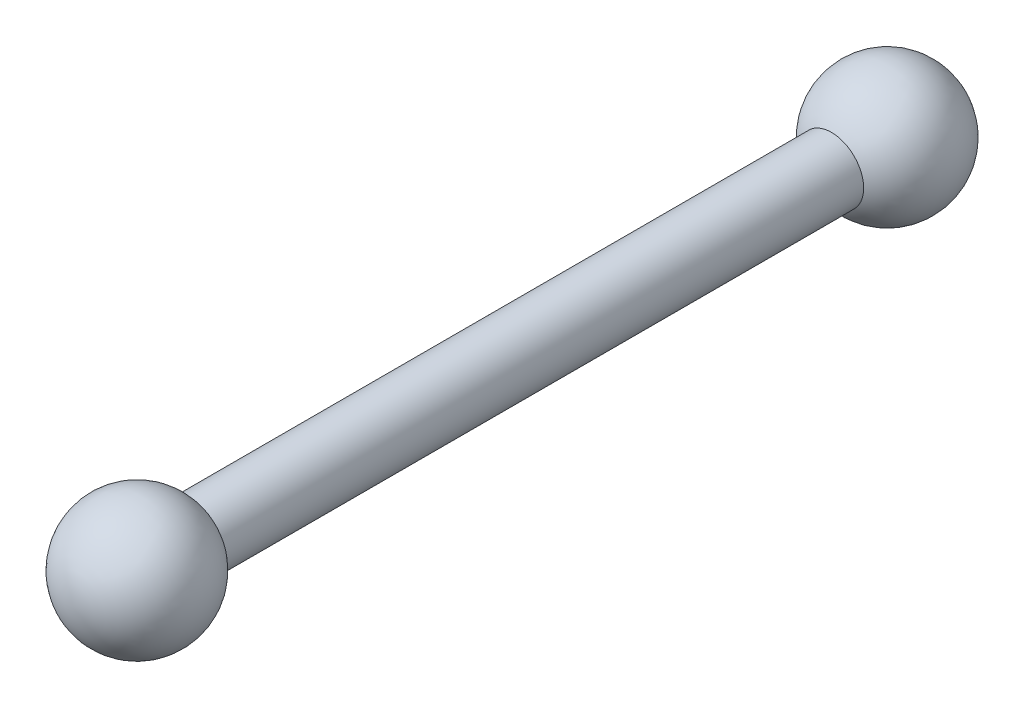
SolidWorks part; units mm, degrees
ref_plane "Front Plane" through (0, 0, 0) normal (0, 0, 1) x (1, 0, 0)
ref_plane "Top Plane" through (0, 0, 0) normal (0, 1, 0) x (1, 0, 0)
ref_plane "Right Plane" through (0, 0, 0) normal (1, 0, 0) x (0, 0, -1)
sketch "Sketch1" plane through (0, 0, 0) normal (0, 0, 1) x (1, 0, 0)
  circle A0 centre (0, 0) radius 15
  dimension "D1" = 30
extrude "Boss-Extrude1" add sketch "Sketch1" along normal mid plane 300
sketch "Sketch2" plane through (0, 0, 0) normal (0, 1, 0) x (1, 0, 0)
  line L0 (0, 205) -> (0, 145)
  line L1 (0, 0) -> (0, 175) construction
  line L2 (15, 150) -> (-15, 150) construction
  arc A0 (0, 145) -> (0, 205) centre (0, 175) ccw
  dimension "D1" = 60
  dimension "D2" = 25
revolve "Revolve1" add sketch "Sketch2" angle 360 about L0
mirror "Mirror1" about plane through (0, 0, 0) normal (0, 0, 1) of "Revolve1"
